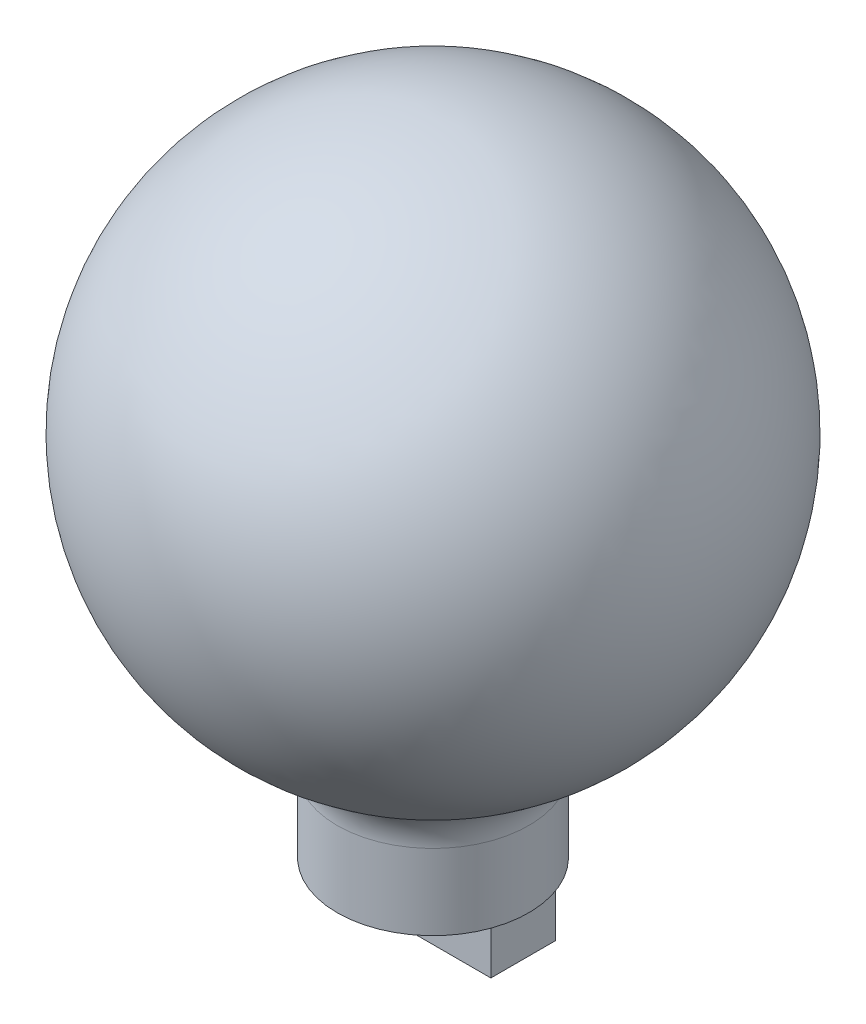
SolidWorks part; units mm, degrees
material "PET"
ref_plane "Front Plane" through (0, 0, 0) normal (0, 0, 1) x (1, 0, 0)
ref_plane "Top Plane" through (0, 0, 0) normal (0, 1, 0) x (1, 0, 0)
ref_plane "Right Plane" through (0, 0, 0) normal (1, 0, 0) x (0, 0, -1)
sketch "Sketch1" plane through (0, 0, 0) normal (0, 0, 1) x (1, 0, 0)
  line L0 (0, 12.7) -> (0, -12.7) construction
  line L1 (0, 12.7) -> (0, -12.7)
  arc A0 (0, 12.7) -> (0, -12.7) centre (0, 0) ccw
  dimension "D1" = 12.7
revolve "Revolve1" add sketch "Sketch1" angle 360 about L0
sketch "Sketch2" plane through (0, 0, 0) normal (0, 0, 1) x (1, 0, 0)
  line L0 (0, 0) -> (-4.445, 0)
  line L1 (-4.445, 0) -> (-4.445, -19.05)
  line L2 (-4.445, -19.05) -> (0, -19.05)
  line L3 (0, -19.05) -> (0, 0) construction
  line L4 (0, 0) -> (0, -19.05)
  circle A0 centre (0, 0) radius 12.7 construction
  dimension "D1" = 4.445
  dimension "D2" = 31.75
revolve "Revolve2" add sketch "Sketch2" angle 360 about L3
fillet "Filete2" radius 2.54 1 edges at (-4.445, -11.8967, 0)
sketch "Sketch3" plane through (0, 0, 0) normal (1, 0, 0) x (0, 0, -1)
  line L1 (-8.89, -24.765) -> (-8.89, -73.025)
  line L2 (-8.89, -73.025) -> (8.89, -73.025)
  line L3 (8.89, -73.025) -> (8.89, -24.765)
  arc A0 (-8.89, -24.765) -> (8.89, -24.765) centre (0, -24.765) cw
  arc A1 (5.8208, -11.2875) -> (-5.8208, -11.2875) centre (0, 0) ccw construction
  dimension "D2" = 8.89
  dimension "D1" = 28.575
  dimension "D3" = 57.15
ref_plane "Plane1" through (0, -23.495, 0) normal (0, 1, 0) x (1, 0, 0)
sketch "Sketch2-T" plane through (0, 0, 0) normal (0, 0, 1) x (1, 0, 0)
  line L0 (-19.05, -27.305) -> (-13.97, -52.705)
  line L2 (-13.97, -52.705) -> (-13.97, -89.1098)
  line L4 (-13.97, -89.1098) -> (-22.5311, -89.1098)
  line L5 (-22.5311, -89.1098) -> (-22.5311, -27.305)
  line L6 (-22.5311, -27.305) -> (-19.05, -27.305)
  line L7 (0, 0) -> (0, -89.38) construction
  line L8 (22.5311, -27.305) -> (19.05, -27.305)
  line L9 (22.5311, -85.8214) -> (22.5311, -27.305)
  line L10 (13.97, -85.8214) -> (22.5311, -85.8214)
  line L11 (13.97, -52.705) -> (13.97, -85.8214)
  line L12 (19.05, -27.305) -> (13.97, -52.705)
sketch "Sketch1-T" plane through (0, 0, 0) normal (1, 0, 0) x (0, 0, -1)
  line L0 (-8.89, -27.305) -> (-6.35, -61.595)
  line L2 (8.89, -27.305) -> (6.35, -61.595)
  line L4 (-6.35, -61.595) -> (-6.35, -73.025)
  line L6 (-6.35, -73.025) -> (6.35, -73.025)
  line L7 (6.35, -73.025) -> (6.35, -61.595)
  line L8 (8.89, -27.305) -> (22.0216, -27.305)
  line L9 (22.0216, -27.305) -> (20.733, -86.5748)
  line L10 (20.733, -86.5748) -> (-27.6828, -86.5748)
  line L11 (-27.6828, -86.5748) -> (-27.6828, -27.305)
  line L12 (-27.6828, -27.305) -> (-8.89, -27.305)
  dimension "D1" = 12.7
sketch "Sketch7-T" plane through (0, 0, 0) normal (1, 0, 0) x (0, 0, -1)
  circle A0 centre (0, -24.765) radius 6.35
  circle A1 centre (0, -66.675) radius 2.5
  dimension "D1" = 12.7
  dimension "D2" = 5
extrude "Cut-Extrude4-T" cut sketch "Sketch7-T" against normal mid plane 50.8
sketch "草图1" plane through (0, 0, 0) normal (1, 0, 0) x (0, 0, -1)
  line L0 (-4.445, -19.05) -> (-2.7679, -19.05) construction
  line L1 (-7.907, -17.05) -> (7.7939, -17.05)
  line L2 (-7.907, -17.05) -> (-7.907, -21.6701)
  line L3 (-7.907, -21.6701) -> (7.7939, -21.6701)
  line L4 (7.7939, -17.05) -> (7.7939, -21.6701)
  dimension "D1" = 2
extrude "Cut-Extrude1" cut sketch "草图1" against normal through all both and the other way through all
sketch "草图2" plane through (0, -17.05, 0) normal (0, -1, 0) x (1, 0, 0)
  line L1 (4.1843, -1.5) -> (-4.1843, -1.5)
  line L2 (4.1843, -1.5) -> (4.1843, 1.5)
  line L3 (4.1843, 1.5) -> (-4.1843, 1.5)
  line L4 (-4.1843, -1.5) -> (-4.1843, 1.5)
  line L5 (4.1843, -1.5) -> (-4.1843, 1.5) construction
  line L6 (4.1843, 1.5) -> (-4.1843, -1.5) construction
  circle A0 centre (0, 0) radius 4.445 construction
  point P0 (0, 0)
  dimension "D1" = 3
extrude "Boss-Extrude1" add sketch "草图2" along normal blind 2 separate body
sketch "Sketch5" plane through (0, 0, 0) normal (1, 0, 0) x (0, 0, -1)
  arc A0 (5.8208, -11.2875) -> (-5.8208, -11.2875) centre (0, 0) ccw construction
  spline S0 degree 3 poles (-16.5147, 10.2387) (-4.6886, 11.3646) (-12.4122, 1.5262) (-10.8894, -5.5753) (-0.735, -19.6733) (-30.1691, 0.8424) (-16.5147, 10.2387) (-4.6886, 11.3646) (-12.4122, 1.5262) knots -0.619704 -0.278904 -0.093311 0 0.1294 0.272525 0.380296 0.721096 0.906689 1 1.1294 1.272525 1.380296 only from (-7.6916, 10.1059) to (-7.6916, 10.1059)
extrude "Cut-Extrude2" [suppressed] cut sketch "Sketch5" against normal through all both and the other way through all
sketch "Sketch7" plane through (0, 0, 0) normal (0, 0, 1) x (1, 0, 0)
  line L0 (0, 0) -> (0, -30.4655) construction
  spline S0 degree 3 poles (-17.6205, -17.8378) (-15.1023, 19.6687) (-6.9145, 0.2545) (-17.6205, -17.8378) (-15.1023, 19.6687) (-6.9145, 0.2545) knots -1 -0.738889 -0.479058 0 0.261111 0.520942 1 1.261111 1.520942 2 only from (-12.7956, 10.1943) to (-12.7956, 10.1943)
  spline S1 degree 3 poles (17.6205, -17.8378) (15.1023, 19.6687) (6.9145, 0.2545) (17.6205, -17.8378) (15.1023, 19.6687) (6.9145, 0.2545) knots -1 -0.738889 -0.479058 0 0.261111 0.520942 1 1.261111 1.520942 2 only from (12.7956, 10.1943) to (12.7956, 10.1943)
sketch "Sketch8" plane through (0, 0, 0) normal (1, 0, 0) x (0, 0, -1)
  line L0 (12.7, 0) -> (-7.6916, 0)
  arc A0 (5.8208, -11.2875) -> (-7.6916, 10.1059) centre (0, 0) ccw construction
scale "Scale1" bodies to scale 130 128 scale about origin uniform scaling yes scale factor 8.6
sketch "Sketch9" plane through (0, 0, 0) normal (1, 0, 0) x (0, 0, -1)
  line L0 (109.22, 0) -> (-62.78, 0)
  line L1 (-62.78, 0) -> (-62.78, 130.243) construction
  arc A0 (50.0592, -97.0726) -> (-50.0592, -97.0726) centre (0, 0) ccw construction
  dimension "D1" = 172
sketch "Sketch10" plane through (0, 0, 0) normal (0, 0, 1) x (1, 0, 0)
  line L0 (-65.5, 52.2727) -> (65.5, 52.2727) construction
  point P2 (0, 52.2727)
  dimension "D1" = 131
ref_plane "Plane1-T" through (0, 0, 62.78) normal (0, 0, 1) x (1, 0, 0)
sketch "Sketch11" plane through (0, 0, 62.78) normal (0, 0, 1) x (1, 0, 0)
  line L0 (-74.7458, 77.0332) -> (-74.7458, 27.5121) construction
  line L1 (-65.5, 52.2727) -> (65.5, 52.2727) construction
  line L2 (0, 0) -> (0, 130.243) construction
  line L3 (-74.7458, 77.0332) -> (-74.7458, 27.5121)
  ellipse E0 centre (-74.7458, 52.2727) end of major axis (-74.7458, 27.5121) minor radius 9.2458 (-74.7458, 27.5121) -> (-74.7458, 77.0332) ccw
  dimension "D1" = 65.5
